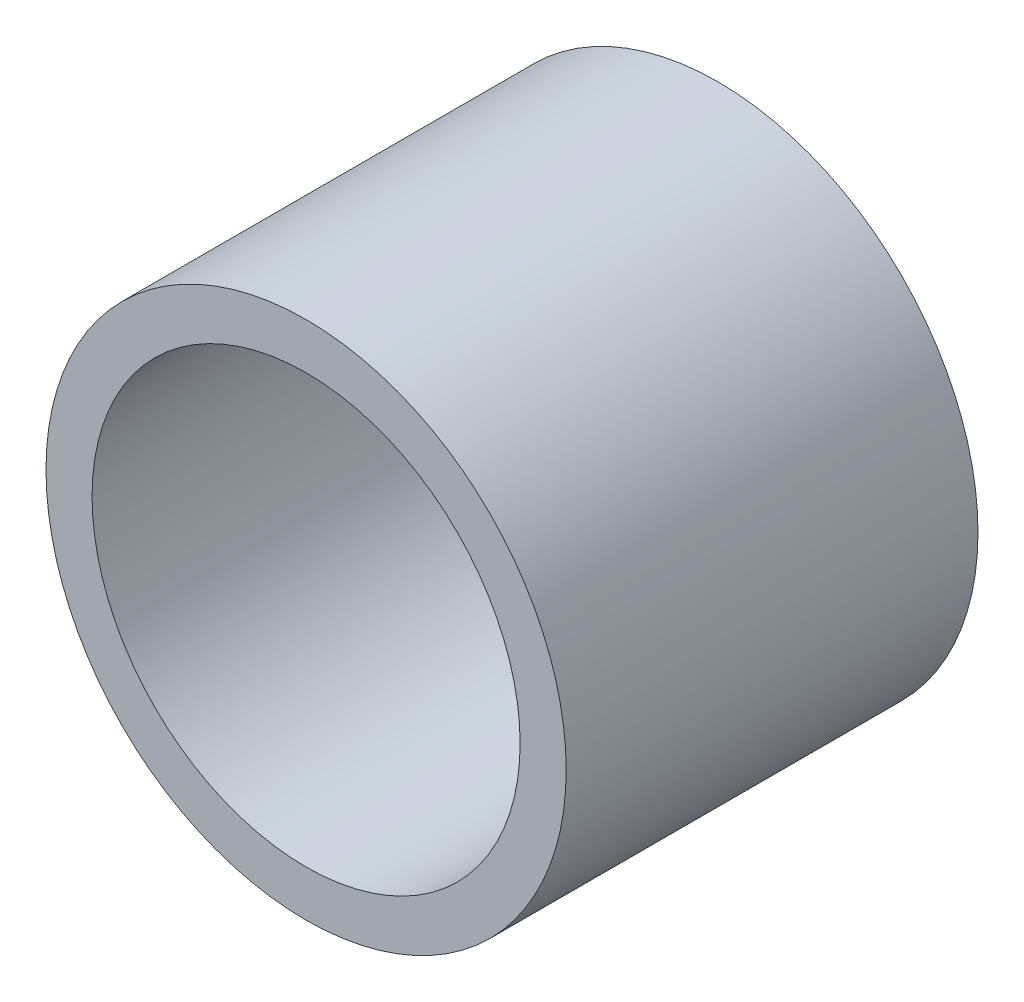
SolidWorks part; units mm, degrees
ref_plane "Front Plane" through (0, 0, 0) normal (0, 0, 1) x (1, 0, 0)
ref_plane "Top Plane" through (0, 0, 0) normal (0, 1, 0) x (1, 0, 0)
ref_plane "Right Plane" through (0, 0, 0) normal (1, 0, 0) x (0, 0, -1)
sketch "Sketch1" plane through (0, 0, 0) normal (0, 0, 1) x (1, 0, 0)
  circle A0 centre (0, 0) radius 24
  circle A1 centre (0, 0) radius 19.75
  dimension "D1" = 48
  dimension "D2" = 39.5
extrude "Boss-Extrude1" add sketch "Sketch1" along normal mid plane 38
